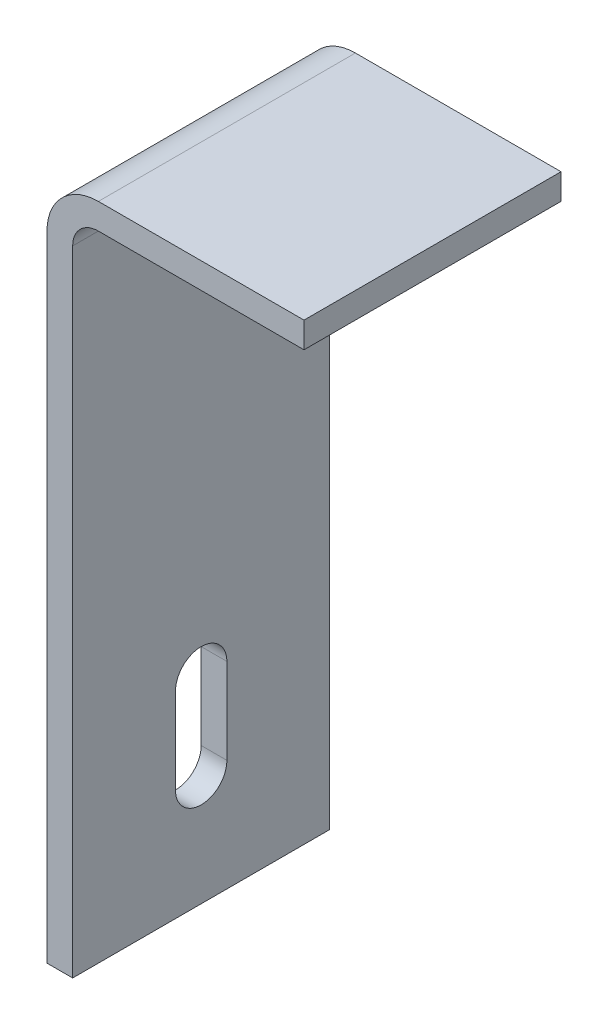
from build123d import *

# Parameters (mm, degrees)
EXTRUDE_THIN1_DEPTH = 30
CUT_EXTRUDE1_DEPTH  = 3


with BuildPart() as part:
    # Sketch1 → Extrude-Thin1 (new body)
    with BuildSketch(Plane.XY):
        with BuildLine():
            Line((0, -80), (0, -6))
            ThreePointArc((0, -6), (1.757359313, -1.757359313), (6, 0))
            Line((6, 0), (30, 0))
            Line((30, 0), (30, -3))
            Line((30, -3), (6, -3))
            ThreePointArc((6, -3), (3.878679656, -3.878679656), (3, -6))
            Line((3, -6), (3, -80))
            Line((3, -80), (0, -80))
        make_face()
    extrude(amount=EXTRUDE_THIN1_DEPTH)

    # Sketch2 → Cut-Extrude1 (cut)
    with BuildSketch(Plane.ZY):
        with BuildLine():
            Line((18, -57), (18, -67))
            ThreePointArc((18, -67), (15, -70), (12, -67))
            Line((12, -67), (12, -57))
            ThreePointArc((12, -57), (15, -54), (18, -57))
        make_face()
    extrude(amount=-CUT_EXTRUDE1_DEPTH, mode=Mode.SUBTRACT)


solid = part.part
